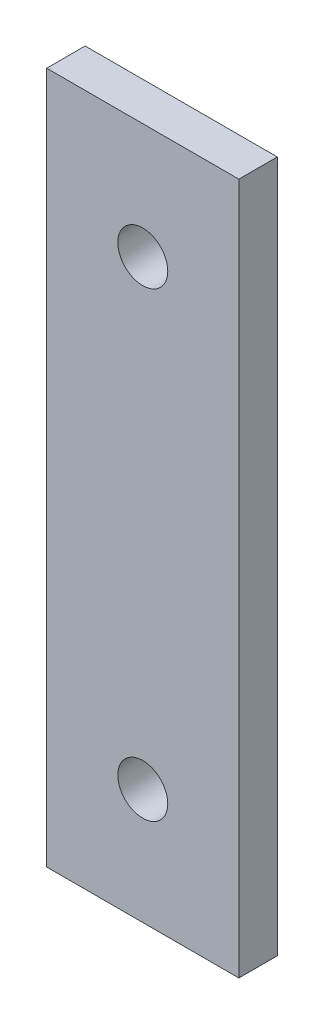
SolidWorks part; units mm, degrees
ref_plane "前视基准面" through (0, 0, 0) normal (0, 0, 1) x (1, 0, 0)
ref_plane "上视基准面" through (0, 0, 0) normal (0, 1, 0) x (1, 0, 0)
ref_plane "右视基准面" through (0, 0, 0) normal (1, 0, 0) x (0, 0, -1)
sketch "草图1" plane through (0, 0, 0) normal (0, 0, 1) x (1, 0, 0)
  line L0 (0, 0) -> (0, 180)
  line L1 (0, 180) -> (50, 180)
  line L2 (50, 180) -> (50, 0)
  line L3 (50, 0) -> (0, 0)
extrude "凸台-拉伸1" add sketch "草图1" along normal blind 10
sketch "草图2" plane through (0, 0, 10) normal (0, 0, 1) x (1, 0, 0)
  line L0 (0, 90) -> (50, 90)
  line L1 (0, 180) -> (0, 0) construction
  line L2 (50, 0) -> (50, 180) construction
  line L3 (25, 90) -> (25, 150)
  line L4 (25, 90) -> (25, 30)
  circle A0 centre (25, 150) radius 6.5
  circle A1 centre (25, 30) radius 6.5
extrude "切除-拉伸1" cut sketch "草图2" against normal blind 10
